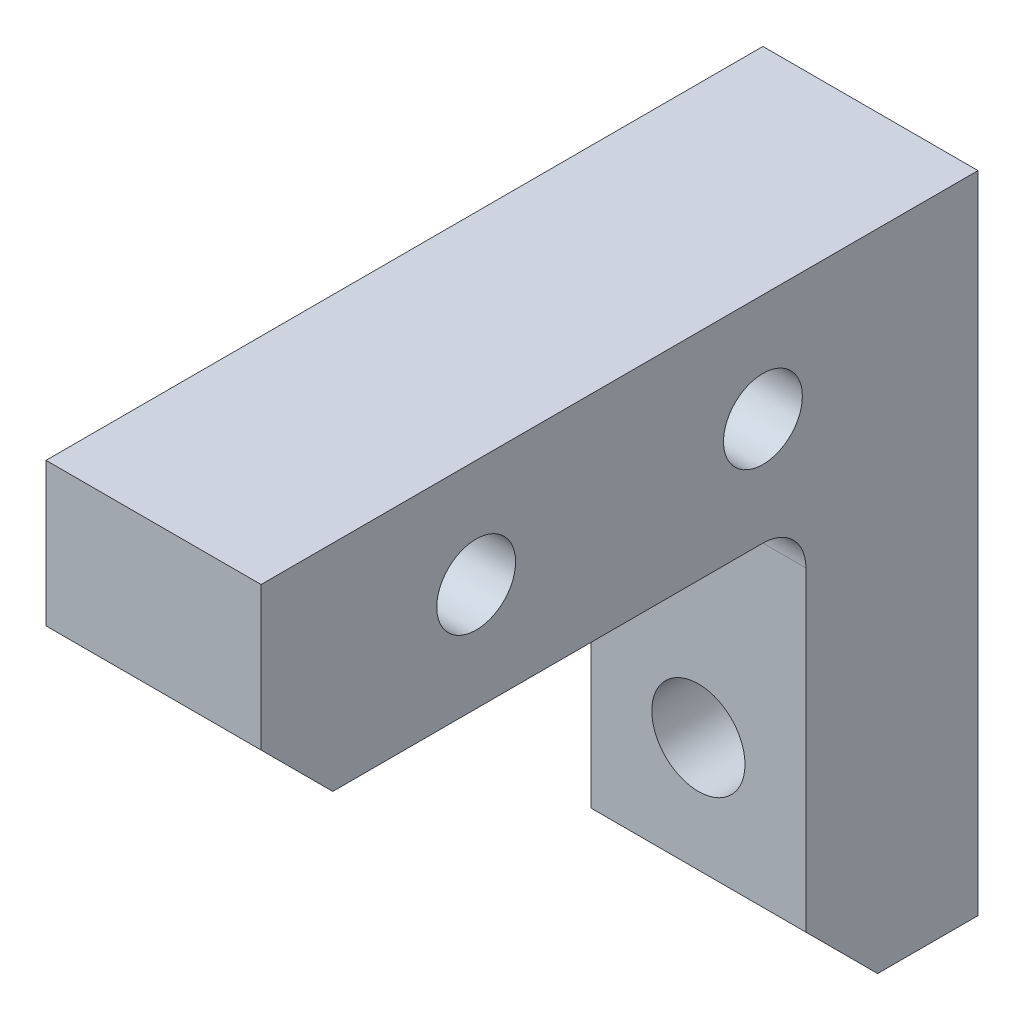
from build123d import *

# Parameters (mm, degrees)
SKETCH_1_W              = 15
SKETCH_1_H              = 15
EXTRUDE_1_DEPTH         = 25
SKETCH_2_W              = 15
SKETCH_2_H              = 30
EXTRUDE_2_DEPTH         = 12
HOLE_WIZARD_6_5_6_5_1_D = 6.5
FILLET_1_R              = 3
CHAMFER_2_SIZE          = 5
HOLE_WIZARD_5_5_5_5_1_D = 5.5


with BuildPart() as part:
    # 草图1 → 凸台-拉伸1 (new, symmetric)
    with BuildSketch(Plane.XY):
        Rectangle(SKETCH_1_W, SKETCH_1_H)
    extrude(amount=EXTRUDE_1_DEPTH, both=True)

    # 草图2 → 凸台-拉伸2 (add)
    with BuildSketch(Plane(origin=(0, 0, -25), x_dir=(-1, 0, 0), z_dir=(0, 0, -1))):
        with Locations((0, -22.5)):
            Rectangle(SKETCH_2_W, SKETCH_2_H)
    extrude(amount=-EXTRUDE_2_DEPTH)

    # Ø6.5 (6.5) 直径孔1 (through all)
    with Locations(Plane.XY.offset(-13)):
        with Locations((0, -24.5)):
            Hole(HOLE_WIZARD_6_5_6_5_1_D / 2)

    # 圆角1
    fillet_1_edges = [part.edges().sort_by_distance(p)[0] for p in [
        (0, -7.5, -13),
    ]]
    fillet(fillet_1_edges, radius=FILLET_1_R)

    # 倒角2
    chamfer_2_edges = [part.edges().sort_by_distance(p)[0] for p in [
        (0, -37.5, -13),
        (0, -7.5, 25),
    ]]
    chamfer(chamfer_2_edges, length=CHAMFER_2_SIZE)

    # Ø5.5 (5.5) 直径孔1 (through all)
    with Locations(Plane(origin=(7.5, 0, 0), x_dir=(0, 0, -1), z_dir=(1, 0, 0))):
        with Locations((10, 0), (-10, 0)):
            Hole(HOLE_WIZARD_5_5_5_5_1_D / 2)


solid = part.part
